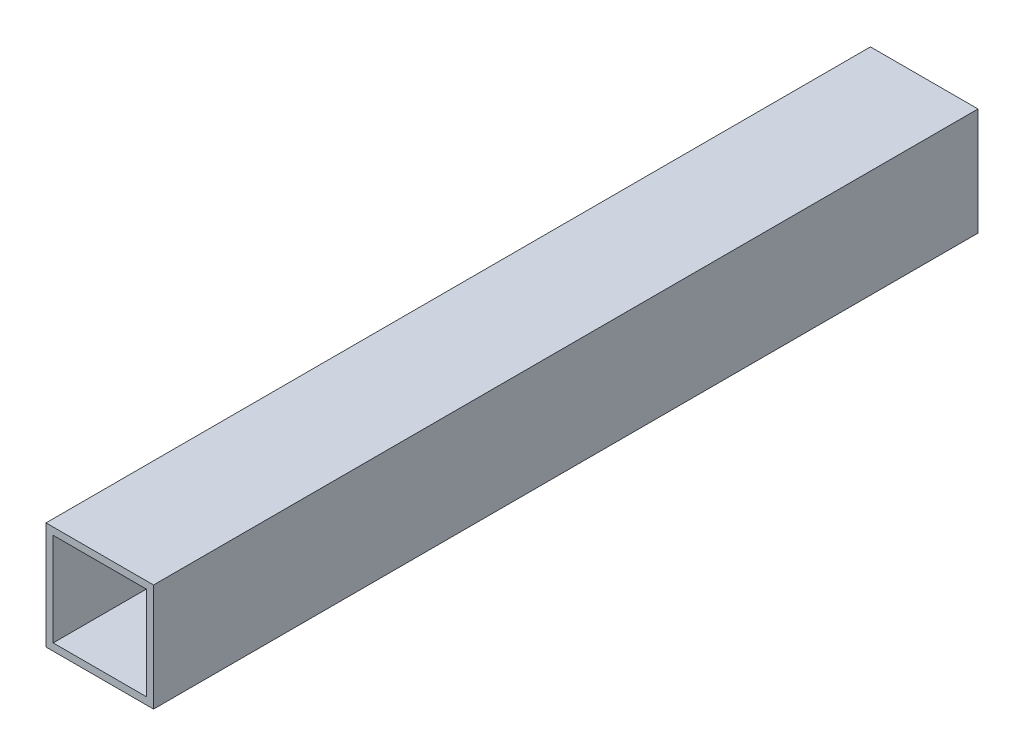
from build123d import *

# Parameters (mm, degrees)
SKETCH_1_W      = 30
SKETCH_1_H      = 30
SKETCH_1_W_2    = 26
SKETCH_1_H_2    = 26
EXTRUDE_1_DEPTH = 115


with BuildPart() as part:
    # 草图1 → 凸台-拉伸1 (new, symmetric)
    with BuildSketch(Plane.XY):
        Rectangle(SKETCH_1_W, SKETCH_1_H)
        Rectangle(SKETCH_1_W_2, SKETCH_1_H_2, mode=Mode.SUBTRACT)
    extrude(amount=EXTRUDE_1_DEPTH, both=True)


solid = part.part
